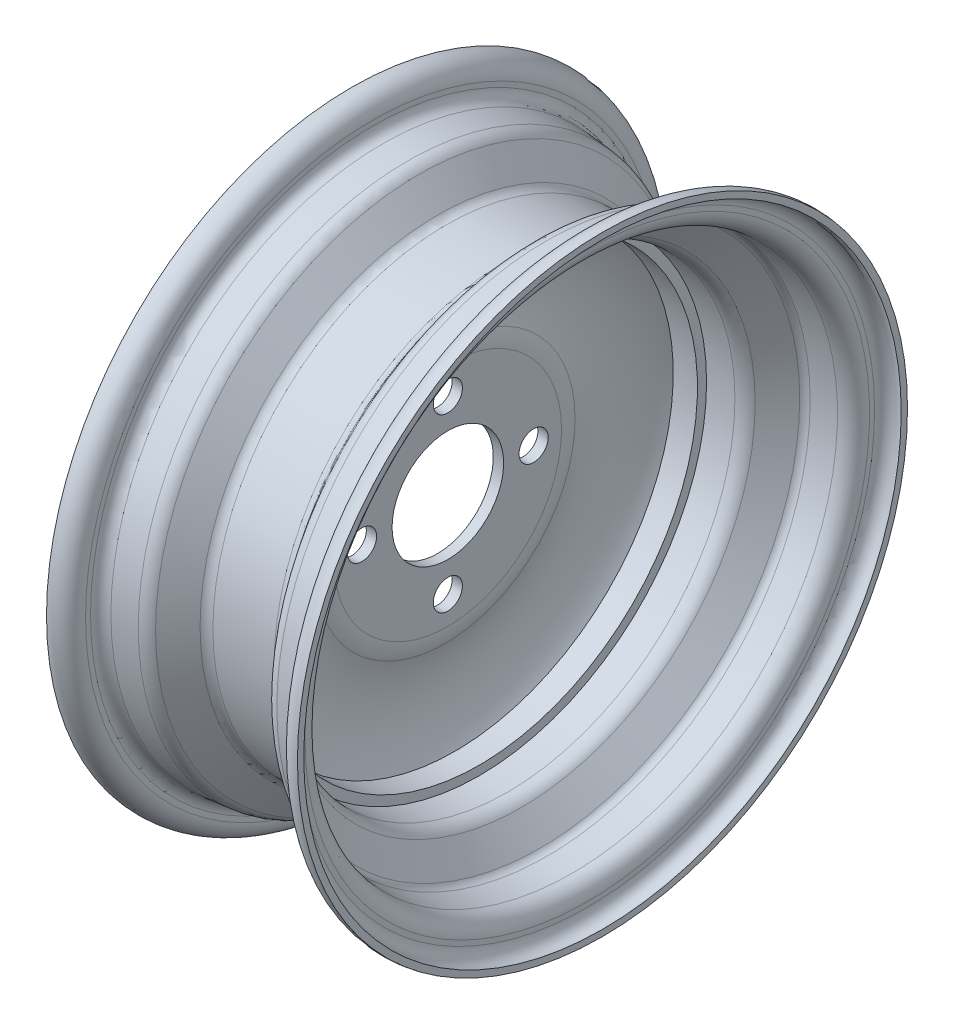
from build123d import *

# Parameters (mm, degrees)
SKETCH_3_R          = 8.5
CUT_EXTRUDE_1_DEPTH = 270.420587168


with BuildPart() as part:
    # 草图2 → 旋转1 (revolve)
    with BuildSketch(Plane.XY, mode=Mode.PRIVATE) as revolve_1_sk:
        with BuildLine():
            Line((55.03343969, 158.353580236), (40.387179575, 157.072222603))
            ThreePointArc((40.387179575, 157.072222603), (36.757353818, 155.957845796), (33.90043136, 153.456753082))
            Line((33.90043136, 153.456753082), (22.81007227, 138.595551029))
            ThreePointArc((22.81007227, 138.595551029), (20.615656314, 136.757442651), (17.830091986, 136.098098151))
            Line((17.830091986, 136.098098151), (-17.830091986, 136.098098151))
            ThreePointArc((-17.830091986, 136.098098151), (-20.615656314, 136.757442651), (-22.81007227, 138.595551029))
            Line((-22.81007227, 138.595551029), (-33.90043136, 153.456753082))
            ThreePointArc((-33.90043136, 153.456753082), (-36.757353818, 155.957845796), (-40.387179575, 157.072222603))
            Line((-40.387179575, 157.072222603), (-55.03343969, 158.353580236))
            ThreePointArc((-55.03343969, 158.353580236), (-59.073188734, 160.345757851), (-60.705705036, 164.543761485))
            Line((-60.705705036, 164.543761485), (-60.705705036, 167.453055254))
            ThreePointArc((-60.705705036, 167.453055254), (-64.495112644, 175.536358254), (-73.132352941, 177.794117647))
            Line((-73.132352941, 177.794117647), (-73.132352941, 174.115893968))
            ThreePointArc((-73.132352941, 174.115893968), (-67.050399463, 172.988692483), (-64.290424508, 167.453055254))
            Line((-64.290424508, 167.453055254), (-64.290424508, 164.543761485))
            ThreePointArc((-64.290424508, 164.543761485), (-61.716119183, 157.923954321), (-55.345862749, 154.782501193))
            Line((-55.345862749, 154.782501193), (-40.699602634, 153.501143561))
            ThreePointArc((-40.699602634, 153.501143561), (-38.50256908, 152.826641973), (-36.773352605, 151.312799441))
            Line((-36.773352605, 151.312799441), (-25.682993515, 136.451597389))
            ThreePointArc((-25.682993515, 136.451597389), (-19.733184391, 132.699966358), (-12.802706935, 133.901401426))
            ThreePointArc((-12.802706935, 133.901401426), (-25.762268543, 106.198547314), (-24.065231305, 75.661382618))
            ThreePointArc((-24.065231305, 75.661382618), (-23.26783219, 72.20191689), (-23, 68.661858362))
            Line((-23, 68.661858362), (-23, 32.5))
            Line((-23, 32.5), (-17, 32.5))
            Line((-17, 32.5), (-17, 66.273791669))
            ThreePointArc((-17, 66.273791669), (-17.379047723, 71.027651805), (-18.506612413, 75.661382618))
            ThreePointArc((-18.506612413, 75.661382618), (-21.261497911, 102.050285854), (-12.802706935, 127.198098151))
            Line((-12.802706935, 127.198098151), (1.3, 127.198098151))
            Line((1.3, 127.198098151), (1.3, 132.513378678))
            Line((1.3, 132.513378678), (17.830091986, 132.513378678))
            ThreePointArc((17.830091986, 132.513378678), (22.222631941, 133.553095131), (25.682993515, 136.451597389))
            Line((25.682993515, 136.451597389), (36.773352605, 151.312799441))
            ThreePointArc((36.773352605, 151.312799441), (38.50256908, 152.826641973), (40.699602634, 153.501143561))
            Line((40.699602634, 153.501143561), (55.345862749, 154.782501193))
            ThreePointArc((55.345862749, 154.782501193), (61.716119183, 157.923954321), (64.290424508, 164.543761485))
            Line((64.290424508, 164.543761485), (64.290424508, 167.453055254))
            ThreePointArc((64.290424508, 167.453055254), (67.050399463, 172.988692483), (73.132352941, 174.115893968))
            Line((73.132352941, 174.115893968), (73.132352941, 177.794117647))
            ThreePointArc((73.132352941, 177.794117647), (64.495112644, 175.536358254), (60.705705036, 167.453055254))
            Line((60.705705036, 167.453055254), (60.705705036, 164.543761485))
            ThreePointArc((60.705705036, 164.543761485), (59.073188734, 160.345757851), (55.03343969, 158.353580236))
        make_face()
    revolve(revolve_1_sk.sketch.rotate(Axis((0, 0, 0), (1, 0, 0)), 90), axis=Axis((0, 0, 0), (1, 0, 0)))

    # 草图3 → 切除-拉伸1 (cut, through all)
    with BuildSketch(Plane.ZY.offset(23)):
        with Locations((0, 50)):
            Circle(SKETCH_3_R)
        with Locations((50, 0)):
            Circle(SKETCH_3_R)
        with Locations((0, -50)):
            Circle(SKETCH_3_R)
        with Locations((-50, 0)):
            Circle(SKETCH_3_R)
    extrude(amount=-CUT_EXTRUDE_1_DEPTH, mode=Mode.SUBTRACT)


solid = part.part
